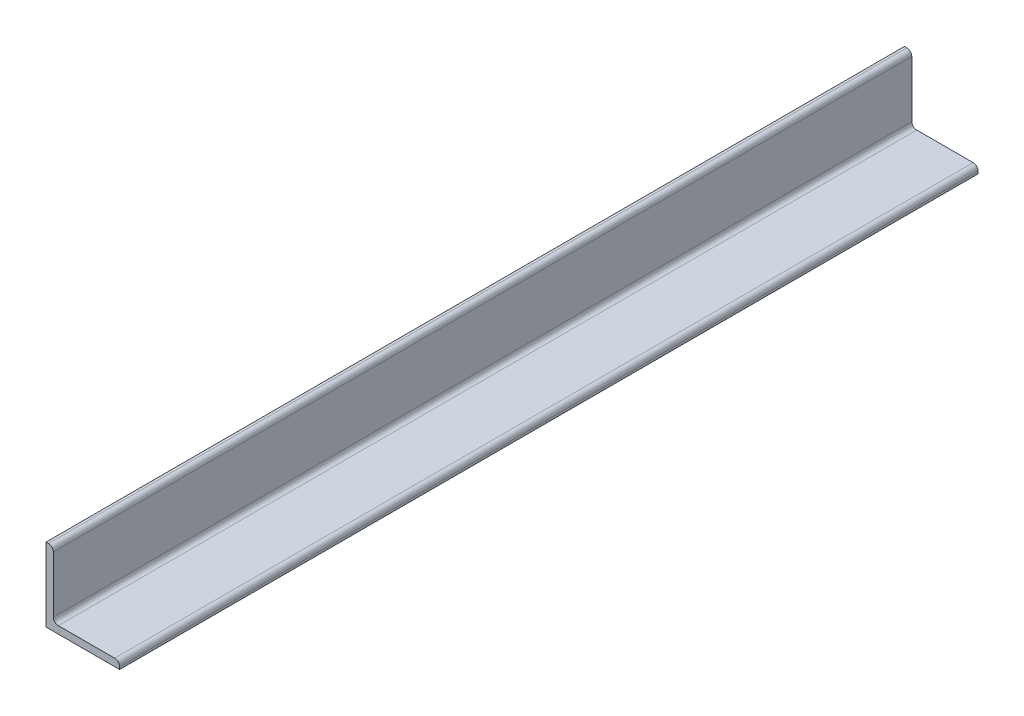
from build123d import *

# Parameters (mm, degrees)
BOSS_EXTRUDE1_DEPTH = 350


with BuildPart() as part:
    # Sketch1 → Boss-Extrude1 (new body)
    with BuildSketch(Plane.XY):
        with BuildLine():
            Line((0, 0), (30, 0))
            Line((30, 0), (30, 1))
            ThreePointArc((30, 1), (29.414213562, 2.414213562), (28, 3))
            Line((28, 3), (5, 3))
            ThreePointArc((5, 3), (3.585786438, 3.585786438), (3, 5))
            Line((3, 5), (3, 28))
            ThreePointArc((3, 28), (2.414213562, 29.414213562), (1, 30))
            Line((1, 30), (0, 30))
            Line((0, 30), (0, 0))
        make_face()
    extrude(amount=BOSS_EXTRUDE1_DEPTH)


solid = part.part
